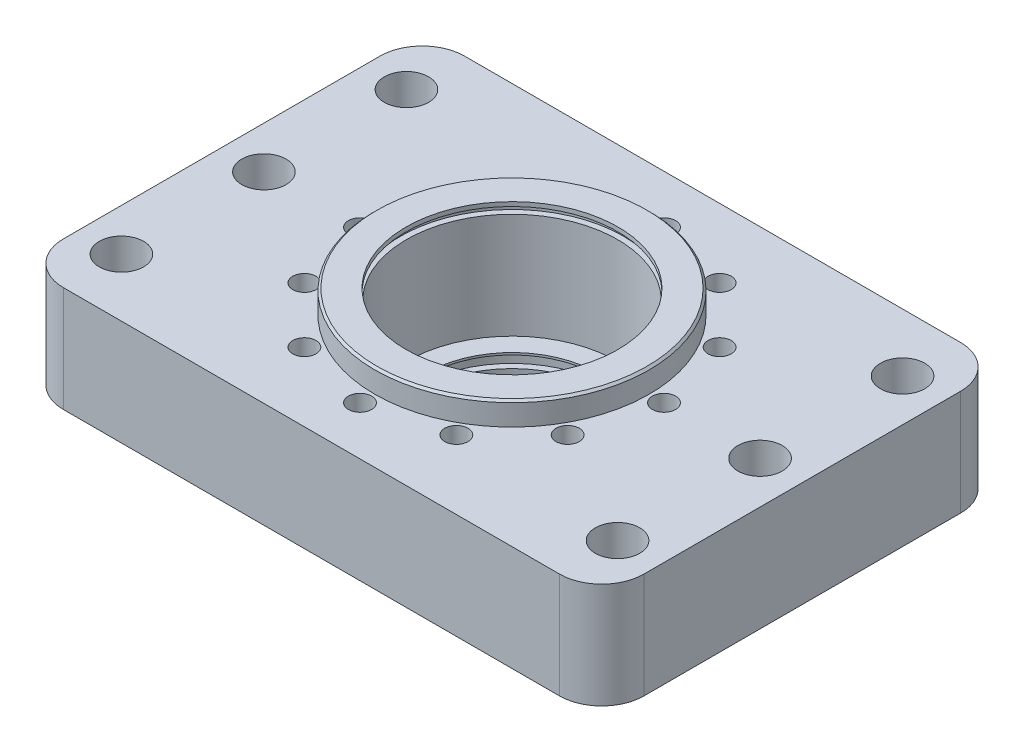
from build123d import *

# Parameters (mm, degrees)
SKETCH1_R                                            = 102.5
BOSS_EXTRUDE1_DEPTH                                  = 50
SKETCH2_R                                            = 65
BOSS_EXTRUDE2_DEPTH                                  = 4
SKETCH3_R                                            = 75
BOSS_EXTRUDE3_DEPTH                                  = 12
CHAMFER1_SIZE                                        = 1
SKETCH4_R                                            = 50
CUT_EXTRUDE1_DEPTH                                   = 55
SKETCH5_R                                            = 40.5
CUT_EXTRUDE2_DEPTH                                   = 156.040317337
CUT_EXTRUDE3_START                                   = -3
SKETCH6_R                                            = 45.5
CUT_EXTRUDE3_DEPTH                                   = 7
SKETCH7_R                                            = 42.5
CUT_EXTRUDE4_DEPTH                                   = 5
CUT_EXTRUDE5_START                                   = -2
SKETCH8_R                                            = 52.75
CUT_EXTRUDE5_DEPTH                                   = 3
SKETCH9_R                                            = 50.25
CUT_EXTRUDE6_DEPTH                                   = 4
HOLE_SIZE_PER_SOCKET_HEAD_CAP_SCREW_TYPE_D           = 11
HOLE_SIZE_PER_SOCKET_HEAD_CAP_SCREW_TYPE_CBORE_D     = 18
HOLE_SIZE_PER_SOCKET_HEAD_CAP_SCREW_TYPE_CBORE_DEPTH = 33
CIRPATTERN1_COUNT                                    = 12
SKETCH14_OUTSIDE_W                                   = 266.466
SKETCH14_OUTSIDE_H                                   = 266.466
SKETCH14_OUTSIDE_R                                   = 82.5
CUT_EXTRUDE7_DEPTH                                   = 20
CHAMFER4_SIZE                                        = 1.5
SKETCH17_R                                           = 5.5
CUT_EXTRUDE11_DEPTH                                  = 151.918852396
CIRPATTERN4_COUNT                                    = 10
M12_TAPPED_HOLE1_D                                   = 10.2
SKETCH22_OUTSIDE_W                                   = 266.466
SKETCH22_OUTSIDE_H                                   = 266.466
SKETCH22_OUTSIDE_R                                   = 82.5
CUT_EXTRUDE12_DEPTH                                  = 155.688396462
SKETCH24_W                                           = 275
SKETCH24_H                                           = 190
SKETCH24_R                                           = 82.5
BOSS_EXTRUDE4_DEPTH                                  = 50
FILLET1_R                                            = 20
MOVE_FACE1_BY                                        = 7
MOVE_FACE2_BY                                        = 7
F_21_0_21_DIAMETER_HOLE1_D                           = 21


with BuildPart() as part:
    # Sketch1 → Boss-Extrude1 (new body)
    with BuildSketch(Plane(origin=(0, 0, 0), x_dir=(1, 0, 0), z_dir=(0, 1, 0))):
        with Locations(Location((0, 0, 0), (0, 0, 270))):
            Circle(SKETCH1_R)
    extrude(amount=BOSS_EXTRUDE1_DEPTH)

    # Sketch2 → Boss-Extrude2 (add)
    with BuildSketch(Plane(origin=(0, 50, 0), x_dir=(1, 0, 0), z_dir=(0, 1, 0))):
        with Locations(Location((0, 0, 0), (0, 0, 270))):
            Circle(SKETCH2_R)
    extrude(amount=BOSS_EXTRUDE2_DEPTH)

    # Sketch3 → Boss-Extrude3 (add)
    with BuildSketch(Plane.XZ):
        with Locations(Location((0, 0, 0), (0, 0, 90))):
            Circle(SKETCH3_R)
    extrude(amount=BOSS_EXTRUDE3_DEPTH)

    # Chamfer1
    chamfer1_edges = [part.edges().sort_by_distance(p)[0] for p in [
        (0, -12, -75),
        (0, 54, -65),
    ]]
    chamfer(chamfer1_edges, length=CHAMFER1_SIZE)

    # Sketch4 → Cut-Extrude1 (cut)
    with BuildSketch(Plane(origin=(0, 54, 0), x_dir=(1, 0, 0), z_dir=(0, 1, 0))):
        with Locations(Location((0, 0, 0), (0, 0, 270))):
            Circle(SKETCH4_R)
    extrude(amount=-CUT_EXTRUDE1_DEPTH, mode=Mode.SUBTRACT)

    # Sketch5 → Cut-Extrude2 (cut, through all)
    with BuildSketch(Plane(origin=(0, -1, 0), x_dir=(1, 0, 0), z_dir=(0, 1, 0))):
        with Locations(Location((0, 0, 0), (0, 0, 270))):
            Circle(SKETCH5_R)
    extrude(amount=-CUT_EXTRUDE2_DEPTH, mode=Mode.SUBTRACT)

    # Sketch6 → Cut-Extrude3 (cut)
    with BuildSketch(Plane.XZ.offset(12).offset(CUT_EXTRUDE3_START)):
        with Locations(Location((0, 0, 0), (0, 0, 270))):
            Circle(SKETCH6_R)
    extrude(amount=-CUT_EXTRUDE3_DEPTH, mode=Mode.SUBTRACT)

    # Sketch7 → Cut-Extrude4 (cut)
    with BuildSketch(Plane.XZ.offset(12)):
        with Locations(Location((0, 0, 0), (0, 0, 270))):
            Circle(SKETCH7_R)
    extrude(amount=-CUT_EXTRUDE4_DEPTH, mode=Mode.SUBTRACT)

    # Sketch8 → Cut-Extrude5 (cut)
    with BuildSketch(Plane(origin=(0, 54, 0), x_dir=(1, 0, 0), z_dir=(0, 1, 0)).offset(CUT_EXTRUDE5_START)):
        with Locations(Location((0, 0, 0), (0, 0, 270))):
            Circle(SKETCH8_R)
    extrude(amount=-CUT_EXTRUDE5_DEPTH, mode=Mode.SUBTRACT)

    # Sketch9 → Cut-Extrude6 (cut)
    with BuildSketch(Plane(origin=(0, 54, 0), x_dir=(1, 0, 0), z_dir=(0, 1, 0))):
        with Locations(Location((0, 0, 0), (0, 0, 270))):
            Circle(SKETCH9_R)
    extrude(amount=-CUT_EXTRUDE6_DEPTH, mode=Mode.SUBTRACT)

    # Hole Size per Socket Head Cap Screw Type1 (through all)
    with Locations(Plane(origin=(0, -12, 0), x_dir=(-1, 0, 0), z_dir=(0, -1, 0))):
        with Locations((0, 72)):
            hole_size_per_socket_head_cap_screw_type = CounterBoreHole(HOLE_SIZE_PER_SOCKET_HEAD_CAP_SCREW_TYPE_D / 2, HOLE_SIZE_PER_SOCKET_HEAD_CAP_SCREW_TYPE_CBORE_D / 2, HOLE_SIZE_PER_SOCKET_HEAD_CAP_SCREW_TYPE_CBORE_DEPTH)

    # CirPattern1: Hole Size per Socket Head Cap Screw Type1 ×12 about axis
    cirpattern1_axis = Axis((0, 0, 0), (0, 1, 0))
    for i in range(1, CIRPATTERN1_COUNT):
        add(hole_size_per_socket_head_cap_screw_type.rotate(cirpattern1_axis, i * 360 / CIRPATTERN1_COUNT), mode=Mode.SUBTRACT)

    # Sketch14 outside → Cut-Extrude7 (cut)
    with BuildSketch(Plane(origin=(0, 50, 0), x_dir=(1, 0, 0), z_dir=(0, 1, 0))):
        Rectangle(SKETCH14_OUTSIDE_W, SKETCH14_OUTSIDE_H)
        with Locations(Location((0, 0, 0), (0, 0, 270))):
            Circle(SKETCH14_OUTSIDE_R, mode=Mode.SUBTRACT)
    extrude(amount=-CUT_EXTRUDE7_DEPTH, mode=Mode.SUBTRACT)

    # Chamfer4
    chamfer4_edges = [part.edges().sort_by_distance(p)[0] for p in [
        (0, 0, -102.5),
        (0, 30, -102.5),
    ]]
    chamfer(chamfer4_edges, length=CHAMFER4_SIZE)

    # Sketch17 → Cut-Extrude11 (cut, through all)
    with BuildSketch(Plane(origin=(0, 30, 0), x_dir=(1, 0, 0), z_dir=(0, 1, 0))):
        with Locations(Location((92.5, 0, 0), (0, 0, 270))):
            Circle(SKETCH17_R)
    cut_extrude11 = extrude(amount=-CUT_EXTRUDE11_DEPTH, mode=Mode.SUBTRACT)

    # CirPattern4: Cut-Extrude11 ×10 about axis
    cirpattern4_axis = Axis((0, 0, 0), (0, 1, 0))
    for i in range(1, CIRPATTERN4_COUNT):
        add(cut_extrude11.rotate(cirpattern4_axis, i * 360 / CIRPATTERN4_COUNT), mode=Mode.SUBTRACT)

    # M12 Tapped Hole1 (through all)
    with Locations(Plane(origin=(0, 0, 0), x_dir=(-1, 0, 0), z_dir=(0, -1, 0))):
        with Locations((-87.972727757, 28.58407198)):
            Hole(M12_TAPPED_HOLE1_D / 2)

    # Sketch22 outside → Cut-Extrude12 (cut, through all)
    with BuildSketch(Plane.XZ):
        Rectangle(SKETCH22_OUTSIDE_W, SKETCH22_OUTSIDE_H)
        with Locations(Location((0, 0, 0), (0, 0, 90))):
            Circle(SKETCH22_OUTSIDE_R, mode=Mode.SUBTRACT)
    extrude(amount=-CUT_EXTRUDE12_DEPTH, mode=Mode.SUBTRACT)

    # Sketch24 → Boss-Extrude4 (add)
    with BuildSketch(Plane.XZ):
        Rectangle(SKETCH24_W, SKETCH24_H)
        Circle(SKETCH24_R, mode=Mode.SUBTRACT)
    extrude(amount=-BOSS_EXTRUDE4_DEPTH)

    # Fillet1
    fillet1_edges = [part.edges().sort_by_distance(p)[0] for p in [
        (-137.5, 25, -95),
        (-137.5, 25, 95),
        (137.5, 25, 95),
        (137.5, 25, -95),
    ]]
    fillet(fillet1_edges, radius=FILLET1_R)

    # Move Face1: a face moved outward by 7.0
    extrude(part.faces().sort_by_distance((-68.75, 0, 47.5))[0], amount=MOVE_FACE1_BY, dir=(0, -1, 0))

    # Move Face2: a face moved inward by 7.0
    extrude(part.faces().sort_by_distance((68.75, 50, -47.5))[0], amount=MOVE_FACE2_BY, dir=(0, -1, 0), mode=Mode.SUBTRACT)

    # Ø21.0 (21) Diameter Hole1 (through all)
    with Locations(Plane(origin=(0, -7, 0), x_dir=(-1, 0, 0), z_dir=(0, -1, 0))):
        with Locations((-117.5, 67.5), (-117.5, 0), (-117.5, -67.5), (117.5, 67.5), (117.5, 0), (117.5, -67.5)):
            Hole(F_21_0_21_DIAMETER_HOLE1_D / 2)


solid = part.part
